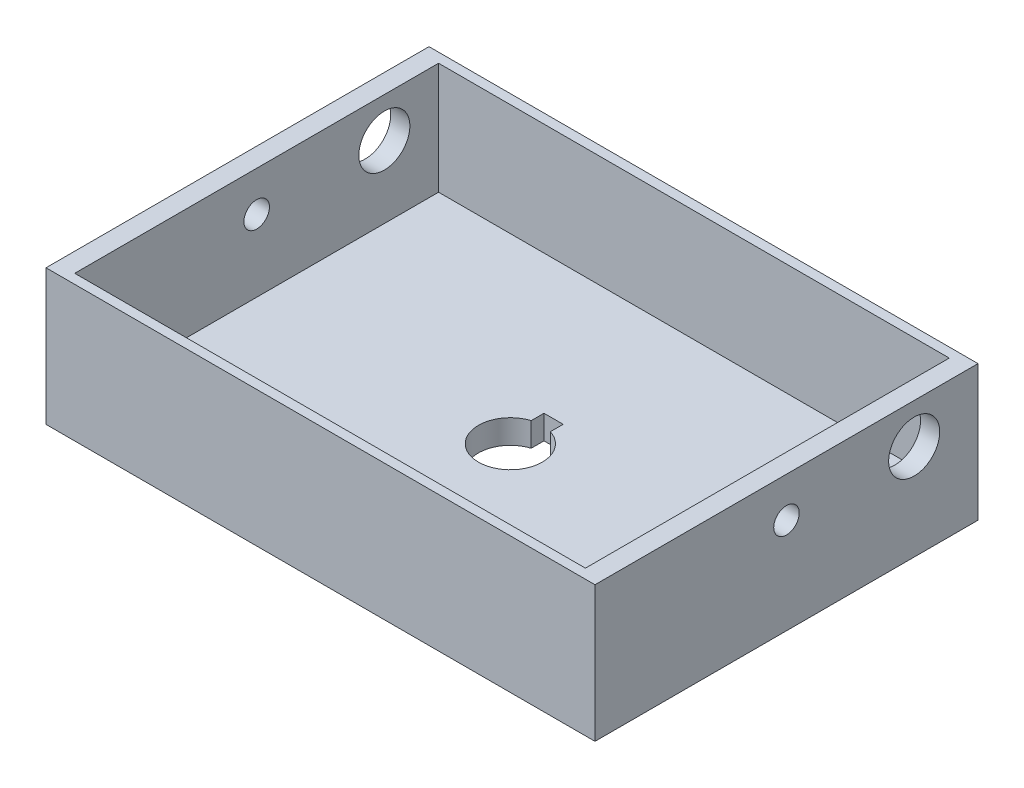
SolidWorks part; units mm, degrees
material "6061-T6 (SS)"
ref_plane "前视基准面" through (0, 0, 0) normal (0, 0, 1) x (1, 0, 0)
ref_plane "上视基准面" through (0, 0, 0) normal (0, 1, 0) x (1, 0, 0)
ref_plane "右视基准面" through (0, 0, 0) normal (1, 0, 0) x (0, 0, -1)
other "Configuration Table"
sketch "草图1" plane through (0, 0, 0) normal (0, 0, 1) x (1, 0, 0)
  line L1 (-86, -21.25) -> (86, -21.25)
  line L2 (-86, -21.25) -> (-86, 21.25)
  line L3 (-86, 21.25) -> (86, 21.25)
  line L4 (86, -21.25) -> (86, 21.25)
  line L5 (-86, -21.25) -> (86, 21.25) construction
  line L6 (-86, 21.25) -> (86, -21.25) construction
  point P0 (0, 0)
  dimension "D1" = 172
  dimension "D2" = 42.5
extrude "凸台-拉伸2" add sketch "草图1" along normal blind 120
sketch "草图2" plane through (0, 21.25, 0) normal (0, 1, 0) x (1, 0, 0)
  line L0 (-80, -5) -> (-80, -3)
  line L3 (-80, -3) -> (80, -3)
  line L4 (80, -3) -> (80, -5)
  line L7 (-80, -5) -> (-80, -117)
  line L8 (-80, -117) -> (80, -117)
  line L9 (80, -5) -> (80, -117)
  dimension "D1" = 2
extrude "切除-拉伸1" cut sketch "草图2" against normal blind 35
sketch "草图5" plane through (-86, 0, 0) normal (-1, 0, 0) x (0, 0, 1)
  circle A0 centre (20, 8.75) radius 8
  circle A1 centre (60, 8.75) radius 4
  dimension "D3" = 16
  dimension "D2" = 8
  dimension "D1" = 40
extrude "切除-拉伸2" cut sketch "草图5" against normal through all
sketch "草图6" plane through (0, -21.25, 0) normal (0, -1, 0) x (1, 0, 0)
  line L3 (-3.5176, 50.4606) -> (-3.5176, 46.4606)
  line L4 (-3.5176, 46.4606) -> (2.4824, 46.4606)
  line L5 (2.4824, 46.4606) -> (2.4824, 50.4606)
  arc A0 (2.4824, 50.4606) -> (-3.5176, 50.4606) centre (-0.5176, 60) ccw
  point P3 (-0.5176, 60)
  dimension "D1" = 20
  dimension "D3" = 4
extrude "切除-拉伸4" cut sketch "草图6" against normal through all
